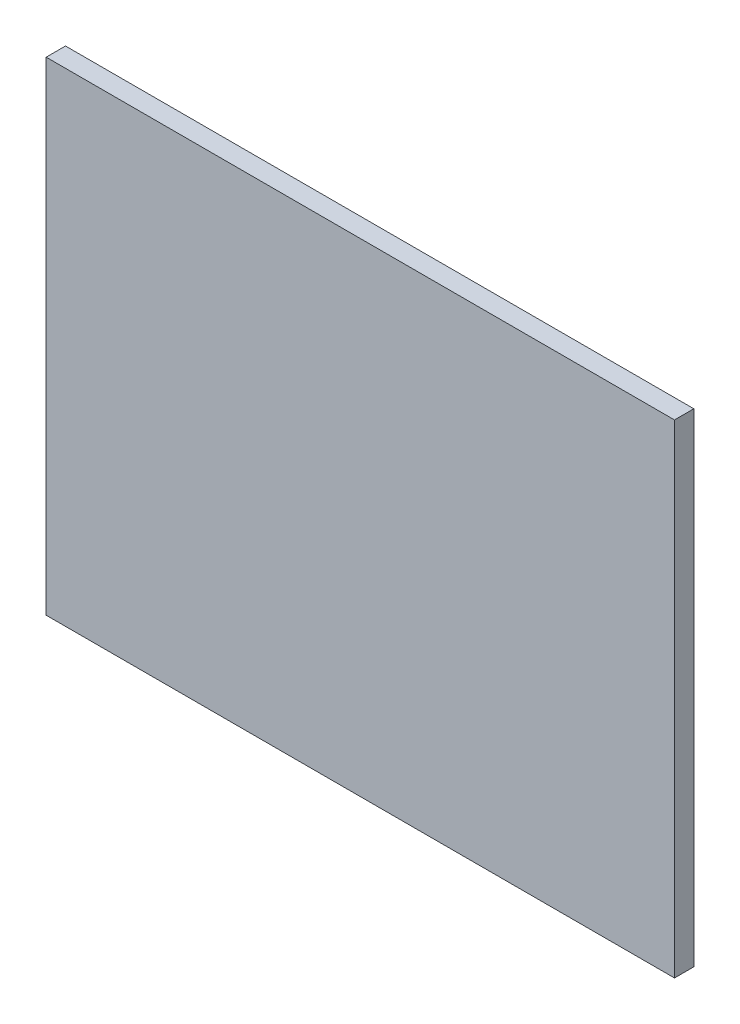
from build123d import *

# Parameters (mm, degrees)
SKETCH1_W           = 390
SKETCH1_H           = 300
BOSS_EXTRUDE1_DEPTH = 12


with BuildPart() as part:
    # Sketch1 → Boss-Extrude1 (new body)
    with BuildSketch(Plane.XY):
        with Locations((195, -150)):
            Rectangle(SKETCH1_W, SKETCH1_H)
    extrude(amount=BOSS_EXTRUDE1_DEPTH)


solid = part.part
